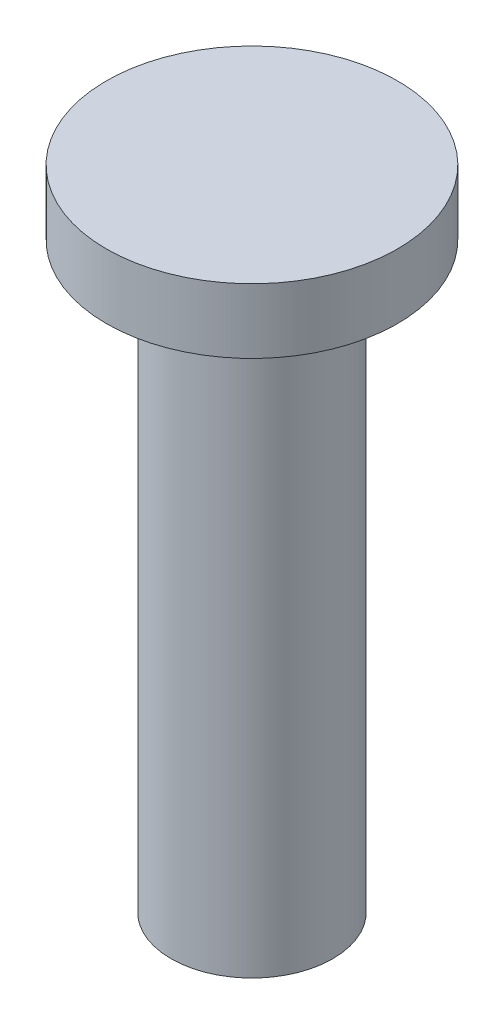
SolidWorks part; units mm, degrees
ref_plane "Front Plane" through (0, 0, 0) normal (0, 0, 1) x (1, 0, 0)
ref_plane "Top Plane" through (0, 0, 0) normal (0, 1, 0) x (1, 0, 0)
ref_plane "Right Plane" through (0, 0, 0) normal (1, 0, 0) x (0, 0, -1)
other "Configuration Table"
sketch "Sketch1" plane through (0, 0, 0) normal (0, 1, 0) x (1, 0, 0)
  circle A0 centre (0, 0) radius 12.5
  dimension "D1" = 25
extrude "Boss-Extrude1" add sketch "Sketch1" along normal blind 100
sketch "Sketch2" plane through (0, 100, 0) normal (0, 1, 0) x (1, 0, 0)
  circle A2 centre (0, 0) radius 22.5
  circle A3 centre (0, 0) radius 22.5
  dimension "D1" = 10
extrude "Boss-Extrude2" add sketch "Sketch2" against normal blind 10
